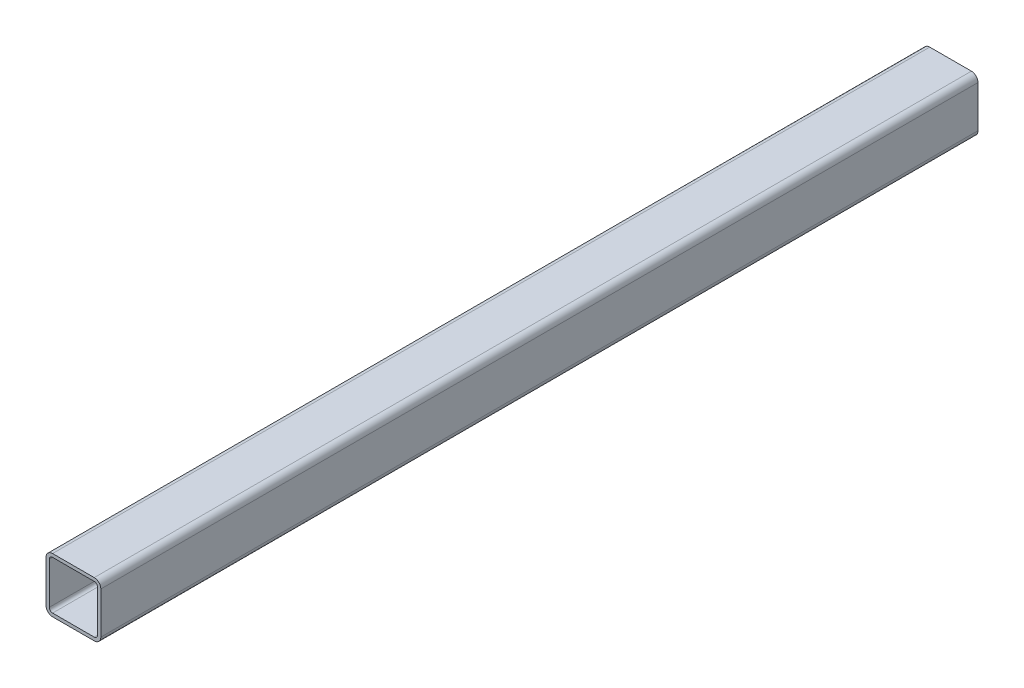
SolidWorks part; units mm, degrees
material "Q235B"
ref_plane "前视基准面" through (0, 0, 0) normal (0, 0, 1) x (1, 0, 0)
ref_plane "上视基准面" through (0, 0, 0) normal (0, 1, 0) x (1, 0, 0)
ref_plane "右视基准面" through (0, 0, 0) normal (1, 0, 0) x (0, 0, -1)
other "Configuration Table"
sketch "草图1" plane through (0, 0, 0) normal (1, 0, 0) x (0, 0, -1)
  line L0 (-400, 0) -> (400, 0)
other "Gb／6728-1986方形空心型钢 050 X 50 X 3(1)"
ref_plane "基准面1" through (0, 0, 400) normal (0, 0, -1) x (0, 1, 0)
sketch "Sketch1" plane through (0, 0, 400) normal (0, 0, -1) x (0, 1, 0)
  line L0 (-19, -22) -> (19, -22)
  line L1 (-22, -19) -> (-22, 19)
  line L2 (19, 22) -> (-19, 22)
  line L3 (22, 19) -> (22, -19)
  line L4 (-19, -25) -> (19, -25)
  line L5 (-25, -19) -> (-25, 19)
  line L6 (19, 25) -> (-19, 25)
  line L7 (25, 19) -> (25, -19)
  arc A0 (25, 19) -> (19, 25) centre (19, 19) ccw
  arc A1 (19, -25) -> (25, -19) centre (19, -19) ccw
  arc A2 (-25, -19) -> (-19, -25) centre (-19, -19) ccw
  arc A3 (-19, 25) -> (-25, 19) centre (-19, 19) ccw
  arc A4 (-19, 22) -> (-22, 19) centre (-19, 19) ccw
  arc A5 (22, 19) -> (19, 22) centre (19, 19) ccw
  arc A6 (19, -22) -> (22, -19) centre (19, -19) ccw
  arc A7 (-22, -19) -> (-19, -22) centre (-19, -19) ccw
  point P0 (-25, 0)
  point P1 (25, 0)
  point P2 (0, 25)
  point P3 (0, -25)
  point P4 (0, 0)
  point P5 (-25, -25)
  point P6 (25, -25)
  point P7 (25, 25)
  point P8 (-25, 25)
  point P33 (0, 0)
  dimension "D1" = 6
  dimension "Thickness" = 3
  dimension "V_leg" = 50
equation "\"D2@草图1\"=\"D1@草图1\"/2"
